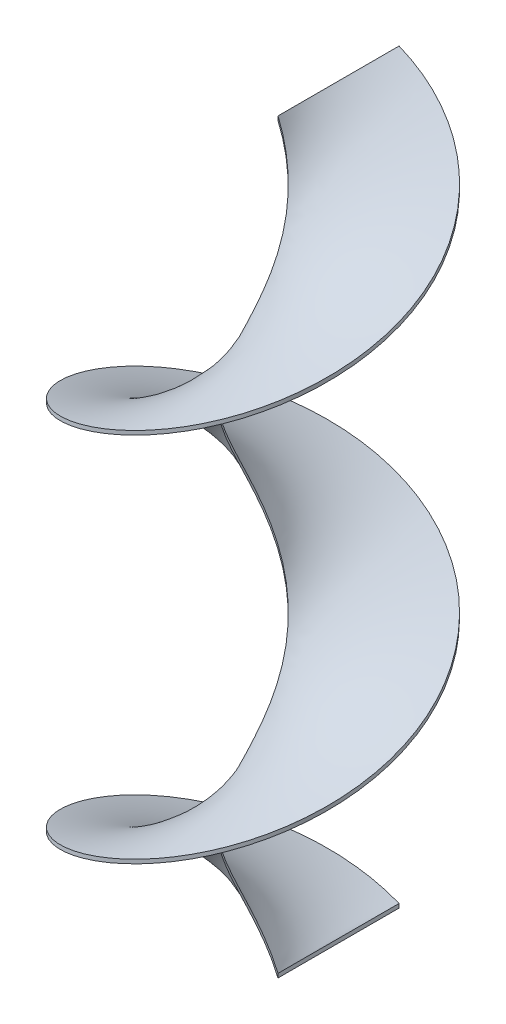
from build123d import *

# Parameters (mm, degrees)
SWEEP_14_PITCH       = 230
SWEEP_14_HEIGHT      = 460
SWEEP_14_RADIUS      = 15
SWEEP_14_START_ANGLE = -180
SKETCH_11_W          = 75
SKETCH_11_H          = 2.5


with BuildPart() as part:
    # 扫描14: sweep along a helix
    with BuildLine() as sweep_14_path:
        add(Helix(SWEEP_14_PITCH, SWEEP_14_HEIGHT, SWEEP_14_RADIUS, center=(0, 0, 0), direction=(0, 1, 0), mode=Mode.PRIVATE).rotate(Axis((0, 0, 0), (0, 1, 0)), SWEEP_14_START_ANGLE))
    # 草图11 → 扫描14 (sweep)
    with BuildSketch(Plane(origin=(0, 0, 0), x_dir=(0, 0, -1), z_dir=(1, 0, 0))):
        with Locations((53, 0)):
            Rectangle(SKETCH_11_W, SKETCH_11_H)
    sweep(path=sweep_14_path.line, is_frenet=True)


solid = part.part
